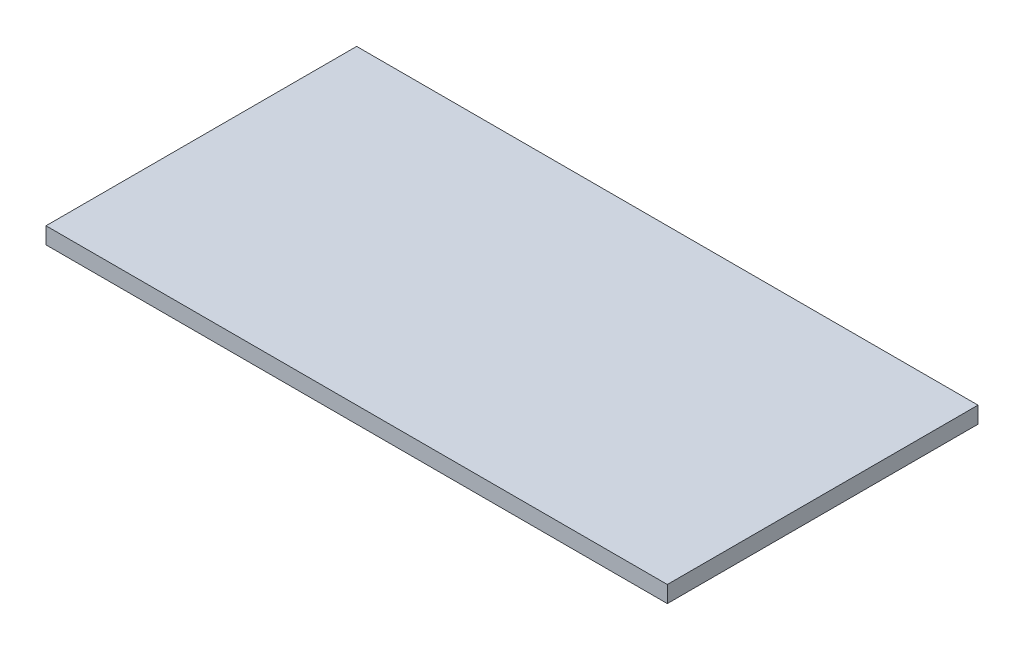
from build123d import *

# Parameters (mm, degrees)
SKETCH1_W           = 600
SKETCH1_H           = 300
BOSS_EXTRUDE1_DEPTH = 20
SKETCH2_OUTSIDE_W   = 736.224
SKETCH2_OUTSIDE_H   = 436.224
SKETCH2_OUTSIDE_W_2 = 580
SKETCH2_OUTSIDE_H_2 = 280
CUT_EXTRUDE1_DEPTH  = 4


with BuildPart() as part:
    # Sketch1 → Boss-Extrude1 (new body)
    with BuildSketch(Plane(origin=(0, 0, 0), x_dir=(1, 0, 0), z_dir=(0, 1, 0))):
        Rectangle(SKETCH1_W, SKETCH1_H)
    extrude(amount=BOSS_EXTRUDE1_DEPTH)

    # Sketch2 outside → Cut-Extrude1 (cut)
    with BuildSketch(Plane.XZ):
        Rectangle(SKETCH2_OUTSIDE_W, SKETCH2_OUTSIDE_H)
        Rectangle(SKETCH2_OUTSIDE_W_2, SKETCH2_OUTSIDE_H_2, mode=Mode.SUBTRACT)
    extrude(amount=-CUT_EXTRUDE1_DEPTH, mode=Mode.SUBTRACT)


solid = part.part
